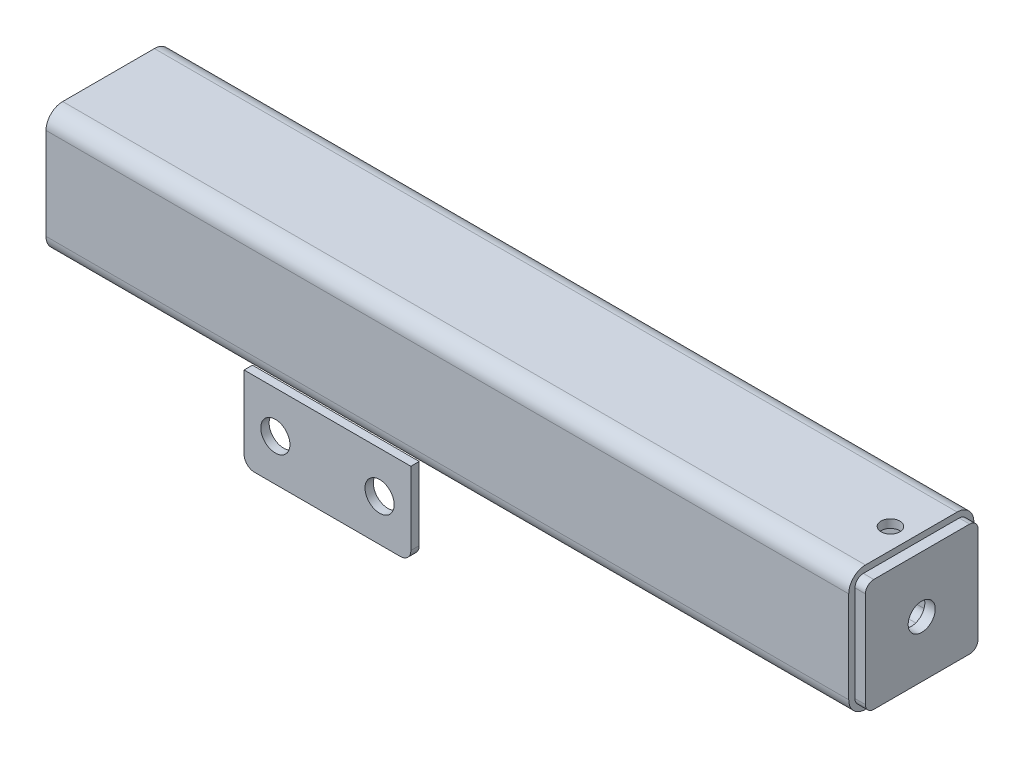
SolidWorks part; units mm, degrees
material "普通碳钢"
ref_plane "前视基准面" through (0, 0, 0) normal (0, 0, 1) x (1, 0, 0)
ref_plane "上视基准面" through (0, 0, 0) normal (0, 1, 0) x (1, 0, 0)
ref_plane "右视基准面" through (0, 0, 0) normal (1, 0, 0) x (0, 0, -1)
sketch "草图1" plane through (0, 0, 0) normal (0, 0, 1) x (1, 0, 0)
  line L0 (0, 0) -> (385, 0)
  dimension "D1" = 385
other "冷弯空心方管gb∕t6728-2002 60 X 60 X 4(1)"
ref_plane "基准面1" through (0, 0, 0) normal (1, 0, 0) x (0, 1, 0)
sketch "Sketch1" plane through (0, 0, 0) normal (1, 0, 0) x (0, 1, 0)
  line L0 (-22, -26) -> (22, -26)
  line L1 (-26, -22) -> (-26, 22)
  line L2 (22, 26) -> (-22, 26)
  line L3 (26, 22) -> (26, -22)
  line L4 (-22, -30) -> (22, -30)
  line L5 (-30, -22) -> (-30, 22)
  line L6 (22, 30) -> (-22, 30)
  line L7 (30, 22) -> (30, -22)
  arc A0 (30, 22) -> (22, 30) centre (22, 22) ccw
  arc A1 (22, -30) -> (30, -22) centre (22, -22) ccw
  arc A2 (-30, -22) -> (-22, -30) centre (-22, -22) ccw
  arc A3 (-22, 30) -> (-30, 22) centre (-22, 22) ccw
  arc A4 (-22, 26) -> (-26, 22) centre (-22, 22) ccw
  arc A5 (26, 22) -> (22, 26) centre (22, 22) ccw
  arc A6 (22, -26) -> (26, -22) centre (22, -22) ccw
  arc A7 (-26, -22) -> (-22, -26) centre (-22, -22) ccw
  point P0 (-30, 0)
  point P1 (30, 0)
  point P2 (0, 30)
  point P3 (0, -30)
  point P4 (0, 0)
  point P5 (-30, -30)
  point P6 (30, -30)
  point P7 (30, 30)
  point P8 (-30, 30)
  point P33 (0, 0)
  dimension "D1" = 8
  dimension "Thickness" = 4
  dimension "V_leg" = 60
sketch "草图3" plane through (385, 0, 0) normal (1, 0, 0) x (0, 0, -1)
  line L0 (26, -22) -> (26, 22) construction
  line L1 (-23, -27) -> (23, -27)
  line L2 (-27, -23) -> (-27, 23)
  line L3 (-23, 27) -> (23, 27)
  line L4 (27, -23) -> (27, 23)
  line L5 (-27, -27) -> (27, 27) construction
  line L6 (-27, 27) -> (27, -27) construction
  line L7 (22, 26) -> (-22, 26) construction
  arc A0 (23, -27) -> (27, -23) centre (23, -23) ccw
  arc A1 (-23, -27) -> (-27, -23) centre (-23, -23) cw
  arc A2 (-27, 23) -> (-23, 27) centre (-23, 23) cw
  arc A3 (23, 27) -> (27, 23) centre (23, 23) cw
  point P0 (0, 0)
  dimension "D3" = 4
  dimension "D1" = 1
  dimension "D2" = 1
extrude "凸台-拉伸1" add sketch "草图3" along normal blind 5 separate body
sketch "草图4" plane through (0, 0, 30) normal (0, 0, 1) x (1, 0, 0)
  line L0 (385, -30) -> (0, -30) construction
  line L1 (175, -30) -> (95, -30)
  line L2 (175, -30) -> (175, -65)
  line L3 (170, -70) -> (100, -70)
  line L4 (95, -30) -> (95, -65)
  line L5 (0, 22) -> (0, -22) construction
  circle A0 centre (110, -50) radius 7
  circle A1 centre (160, -50) radius 7
  arc A2 (175, -65) -> (170, -70) centre (170, -65) cw
  arc A3 (100, -70) -> (95, -65) centre (100, -65) cw
  point P12 (135, -70)
  point P19 (175, -70)
  point P22 (95, -70)
  dimension "D6" = 14
  dimension "D7" = 20
  dimension "D8" = 20
  dimension "D9" = 5
  dimension "D1" = 95
  dimension "D2" = 40
  dimension "D3" = 80
  dimension "D4" = 50
  dimension "D5" = 25
extrude "凸台-拉伸2" add sketch "草图4" against normal blind 4 separate body
mirror "镜向2" about plane through (0, 0, 0) normal (0, 0, 1) of bodies 108
sketch "草图5" plane through (390, 0, 0) normal (1, 0, 0) x (0, 0, -1)
  circle A0 centre (0, 0) radius 6.5
  dimension "D1" = 13
extrude "切除-拉伸1" cut sketch "草图5" against normal blind 5
hole_wizard "M10x1.0 螺纹孔1" positions "草图7" profile "草图8" tap size "M10x1.0" standard "GB"
sketch "草图7" plane through (0, 30, 0) normal (0, 1, 0) x (1, 0, 0)
  line L0 (390, 23) -> (390, -23) construction
  line L1 (385, 30) -> (0, 30) construction
  point P0 (375, 0)
  dimension "D1" = 15
  dimension "D2" = 30
sketch "草图8" plane through (375, 30, 0) normal (1, 0, 0) x (0, 0, 1)
  line L0 (0, 0) -> (0, 10.7039)
  line L1 (0, 10.7039) -> (4.5, 8)
  line L2 (4.5, 8) -> (4.5, 0)
  line L5 (4.5, 0) -> (0, 0)
  line L10 (0, 10.7039) -> (-4.5, 8) construction
  line L11 (0, -6.35) -> (0, 107.95) construction
  dimension "螺纹孔钻头直径" = 9
  dimension "螺纹孔钻头深度" = 8
  dimension "导头角度" = 118
cosmetic thread "孔螺蚊线1"
